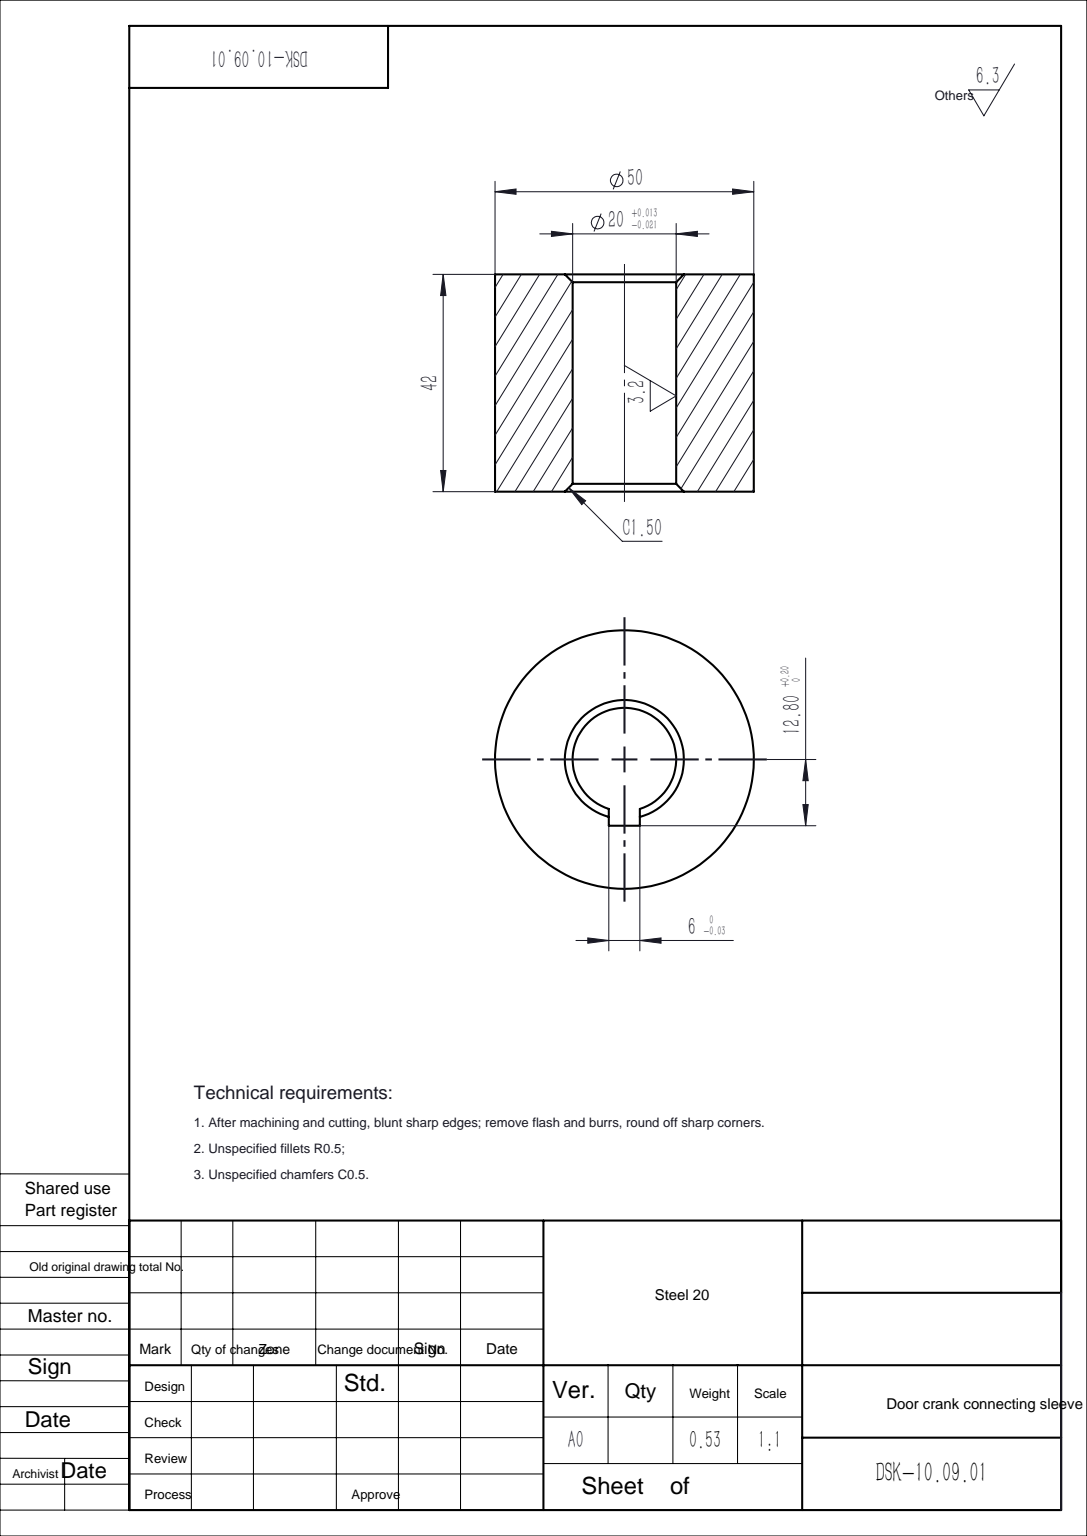
SolidWorks part; units mm, degrees
material "20 steel"
ref_plane "Front Plane" through (0, 0, 0) normal (0, 0, 1) x (1, 0, 0)
ref_plane "Top Plane" through (0, 0, 0) normal (0, 1, 0) x (1, 0, 0)
ref_plane "Right Plane" through (0, 0, 0) normal (1, 0, 0) x (0, 0, -1)
sketch "Sketch1" plane through (0, 0, 0) normal (0, 1, 0) x (1, 0, 0)
  line L1 (3, -7.2) -> (-3, -7.2)
  line L2 (3, -7.2) -> (3, -12.8)
  line L3 (3, -12.8) -> (-3, -12.8)
  line L4 (-3, -7.2) -> (-3, -12.8)
  line L5 (3, -7.2) -> (-3, -12.8) construction
  line L6 (3, -12.8) -> (-3, -7.2) construction
  circle A0 centre (0, 0) radius 25
  circle A1 centre (0, 0) radius 10
  point P4 (0, -10)
  dimension "D1" = 50
  dimension "D2" = 20
  dimension "D3" = 6
  dimension "D4" = 12.8
extrude "Boss-Extrude1" add sketch "Sketch1" along normal blind 42 contours A0 A1 L2 L3 L4
chamfer "Chamfer1" distance 1.5 angle 45 2 edges at (0, 42, -10) (0, 0, -10)
